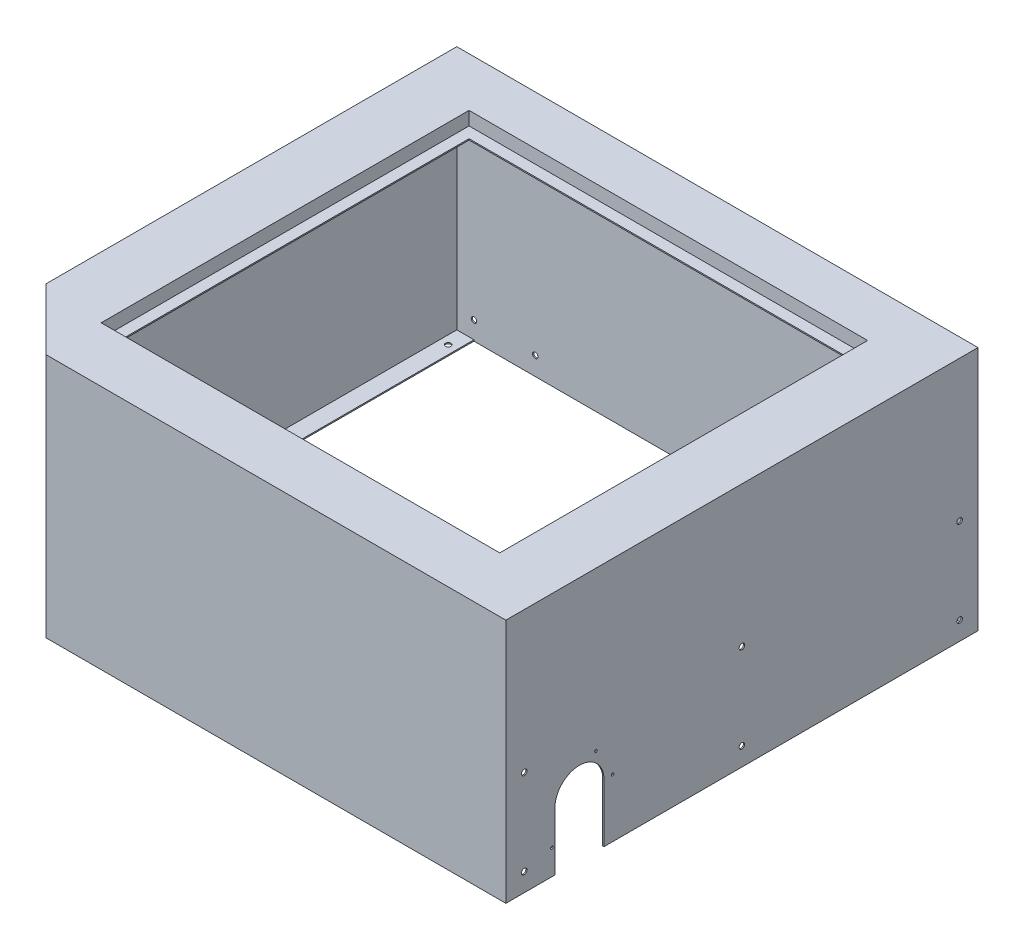
from build123d import *

# Parameters (mm, degrees)
EXTRUDE_1_DEPTH        = 400
SHELL_1_T              = -2
SKETCH_3_W             = 650
SKETCH_3_H             = 600
CUT_EXTRUDE_1_DEPTH    = 2
SKETCH_4_W             = 654
SKETCH_4_H             = 604
SKETCH_4_W_2           = 650
SKETCH_4_H_2           = 600
EXTRUDE_2_DEPTH        = 24
SKETCH_5_W             = 654
SKETCH_5_H             = 604
SKETCH_5_W_2           = 614
SKETCH_5_H_2           = 564
EXTRUDE_3_DEPTH        = 2
EXTRUDE_4_DEPTH        = 2
CUT_EXTRUDE_2_DEPTH    = 2
SKETCH_10_W            = 666
SKETCH_10_H            = 2
EXTRUDE_7_DEPTH        = 28
SKETCH_12_R            = 4.5
CUT_EXTRUDE_3_DEPTH    = 10
SKETCH_13_R            = 4.5
CUT_EXTRUDE_4_DEPTH    = 10
SKETCH_14_R            = 4.5
CUT_EXTRUDE_5_DEPTH    = 10
HOLE_WIZARD_M5_1_D     = 4.2
HOLE_WIZARD_M5_1_DEPTH = 3
HOLE_WIZARD_M5_1_TIP   = 1.2618073


with BuildPart() as part:
    # 草图1 → 凸台-拉伸1 (new body)
    with BuildSketch(Plane(origin=(0, 0, 0), x_dir=(1, 0, 0), z_dir=(0, 1, 0))):
        Polygon((-425, 380), (-425, -290), (-325, -390), (425, -390), (425, 380), align=None)
    extrude(amount=-EXTRUDE_1_DEPTH)

    # 抽壳1
    shell_1_openings = [part.faces().sort_by_distance(p)[0] for p in [
        (3.015139851, -400, 2.292789325),
    ]]
    offset(amount=SHELL_1_T, openings=shell_1_openings, kind=Kind.INTERSECTION)

    # 草图3 → 切除-拉伸1 (cut)
    with BuildSketch(Plane(origin=(0, 0, 0), x_dir=(1, 0, 0), z_dir=(0, 1, 0))):
        Rectangle(SKETCH_3_W, SKETCH_3_H)
    extrude(amount=-CUT_EXTRUDE_1_DEPTH, mode=Mode.SUBTRACT)

    # 草图4 → 凸台-拉伸2 (add)
    with BuildSketch(Plane(origin=(0, 0, 0), x_dir=(1, 0, 0), z_dir=(0, 1, 0))):
        Rectangle(SKETCH_4_W, SKETCH_4_H)
        Rectangle(SKETCH_4_W_2, SKETCH_4_H_2, mode=Mode.SUBTRACT)
    extrude(amount=-EXTRUDE_2_DEPTH)

    # 草图5 → 凸台-拉伸3 (add)
    with BuildSketch(Plane.XZ.offset(24)):
        Rectangle(SKETCH_5_W, SKETCH_5_H)
        Rectangle(SKETCH_5_W_2, SKETCH_5_H_2, mode=Mode.SUBTRACT)
    extrude(amount=-EXTRUDE_3_DEPTH)

    # 草图6 → 凸台-拉伸4 (add)
    with BuildSketch(Plane.XZ.offset(400)):
        Polygon((-425, 290), (-325, 390), (425, 390), (425, 360), (-312.573593129, 360), (-403.786796564, 268.786796564), align=None)
    extrude(amount=-EXTRUDE_4_DEPTH)

    # 草图7 → 切除-拉伸2 (cut)
    with BuildSketch(Plane(origin=(425, 0, 0), x_dir=(0, 0, -1), z_dir=(1, 0, 0))):
        with BuildLine():
            Line((-310, -400), (-310, -305))
            ThreePointArc((-310, -305), (-270, -265), (-230, -305))
            Line((-230, -305), (-230, -400))
            Line((-230, -400), (-310, -400))
        make_face()
    extrude(amount=-CUT_EXTRUDE_2_DEPTH, mode=Mode.SUBTRACT)

    # 草图10 → 凸台-拉伸7 (add)
    with BuildSketch(Plane(origin=(-423, 0, 0), x_dir=(0, 0, -1), z_dir=(1, 0, 0))):
        with Locations((45, -399)):
            Rectangle(SKETCH_10_W, SKETCH_10_H)
    extrude(amount=EXTRUDE_7_DEPTH)

    # 草图12 → 切除-拉伸3 (cut)
    with BuildSketch(Plane(origin=(0, -398, 0), x_dir=(1, 0, 0), z_dir=(0, 1, 0))):
        with Locations(Location((-409, 350, 0), (0, 0, 270))):
            Circle(SKETCH_12_R)
        with Locations(Location((-363.686291501, -328.686291501, 0), (0, 0, 270))):
            Circle(SKETCH_12_R)
        with Locations(Location((-85, -374, 0), (0, 0, 270))):
            Circle(SKETCH_12_R)
        with Locations(Location((395, -374, 0), (0, 0, 270))):
            Circle(SKETCH_12_R)
        with Locations(Location((-409, -90, 0), (0, 0, 270))):
            Circle(SKETCH_12_R)
        with Locations(Location((-25, -374, 0), (0, 0, 270))):
            Circle(SKETCH_12_R)
        with Locations(Location((-409, -150, 0), (0, 0, 270))):
            Circle(SKETCH_12_R)
        with Locations(Location((23, -374, 0), (0, 0, 270))):
            Circle(SKETCH_12_R)
        with Locations(Location((123, -374, 0), (0, 0, 270))):
            Circle(SKETCH_12_R)
    extrude(amount=-CUT_EXTRUDE_3_DEPTH, mode=Mode.SUBTRACT)

    # 草图13 → 切除-拉伸4 (cut)
    with BuildSketch(Plane.XY.offset(-378)):
        with Locations((0, -30)):
            Circle(SKETCH_13_R)
        with Locations((-295, -30)):
            Circle(SKETCH_13_R)
        with Locations((0, -370)):
            Circle(SKETCH_13_R)
        with Locations((-295, -370)):
            Circle(SKETCH_13_R)
        with Locations((-395, -30)):
            Circle(SKETCH_13_R)
        with Locations((-395, -370)):
            Circle(SKETCH_13_R)
        with Locations(Location((295, -30, 0), (0, 0, 180))):
            Circle(SKETCH_13_R)
        with Locations(Location((295, -370, 0), (0, 0, 180))):
            Circle(SKETCH_13_R)
        with Locations(Location((395, -370, 0), (0, 0, 180))):
            Circle(SKETCH_13_R)
        with Locations(Location((395, -30, 0), (0, 0, 180))):
            Circle(SKETCH_13_R)
    extrude(amount=-CUT_EXTRUDE_4_DEPTH, mode=Mode.SUBTRACT)

    # 草图14 → 切除-拉伸5 (cut)
    with BuildSketch(Plane(origin=(425, 0, 0), x_dir=(0, 0, -1), z_dir=(1, 0, 0))):
        with Locations((-360, -230)):
            Circle(SKETCH_14_R)
        with Locations((-360, -370)):
            Circle(SKETCH_14_R)
        with Locations((-5, -230)):
            Circle(SKETCH_14_R)
        with Locations((-5, -370)):
            Circle(SKETCH_14_R)
        with Locations((350, -370)):
            Circle(SKETCH_14_R)
        with Locations((350, -230)):
            Circle(SKETCH_14_R)
    extrude(amount=-CUT_EXTRUDE_5_DEPTH, mode=Mode.SUBTRACT)

    # M5 螺纹孔1
    with Locations(Plane(origin=(425, 0, 0), x_dir=(0, 0, -1), z_dir=(1, 0, 0))):
        with Locations((-243, -258.234628196), (-216, -305), (-315, -359)):
            Hole(HOLE_WIZARD_M5_1_D / 2, depth=HOLE_WIZARD_M5_1_DEPTH)
            with Locations((0, 0, -(HOLE_WIZARD_M5_1_DEPTH + HOLE_WIZARD_M5_1_TIP / 2))):  # 118° drill point
                Cone(0, HOLE_WIZARD_M5_1_D / 2, HOLE_WIZARD_M5_1_TIP, mode=Mode.SUBTRACT)


solid = part.part
